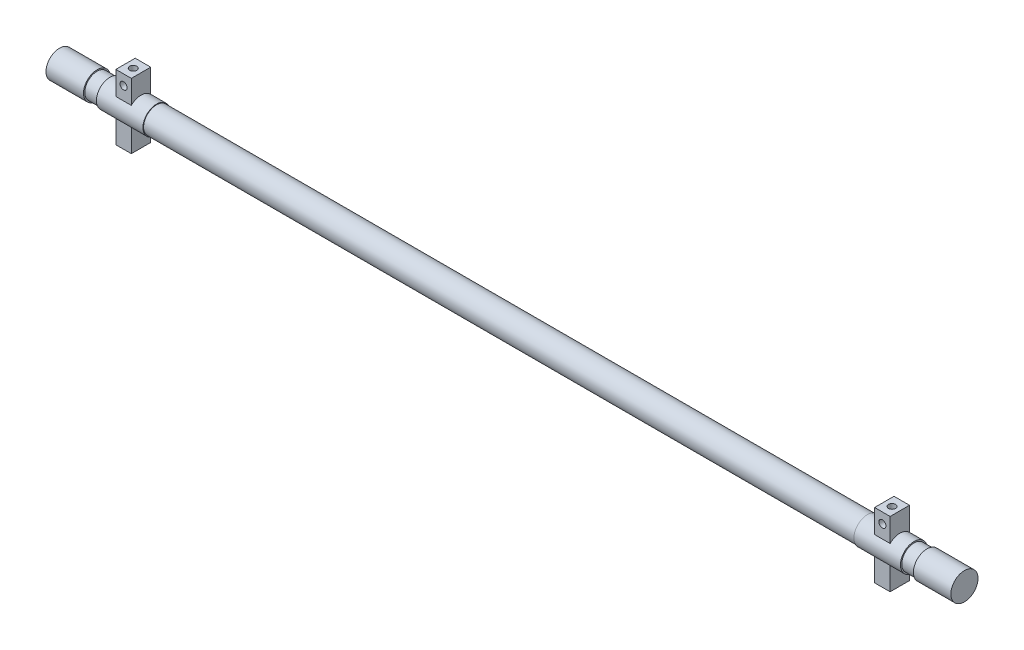
from build123d import *

# Parameters (mm, degrees)
SKETCH2_W            = 12
SKETCH2_H            = 35.5
BOSS_EXTRUDE1_DEPTH  = 7.5
LPATTERN1_COUNT      = 2
LPATTERN1_PITCH      = 587
BOSS_EXTRUDE2_DEPTH  = 15
M5_CLEARANCE_HOLE1_D = 5.5
M5_CLEARANCE_HOLE2_D = 5.5


with BuildPart() as part:
    # Sketch1 → Revolve1 (revolve)
    with BuildSketch(Plane.XY):
        Polygon((0, 0), (0, 10.5), (29, 10.5), (29, 9.5), (39, 9.5), (39, 10.5), (75, 10.5), (75, 10), (625, 10), (625, 10.5), (661, 10.5), (661, 9.5), (671, 9.5), (671, 10.5), (700, 10.5), (700, 0), align=None)
    revolve(axis=Axis((700, 0, 0), (-1, 0, 0)))

    # Sketch2 → Boss-Extrude1 (add, symmetric)
    with BuildSketch(Plane.XY):
        with Locations((57, -7.25)):
            Rectangle(SKETCH2_W, SKETCH2_H)
    boss_extrude1 = extrude(amount=BOSS_EXTRUDE1_DEPTH, both=True)

    # LPattern1: Boss-Extrude1 ×2
    with Locations(*[(i * LPATTERN1_PITCH, 0, 0) for i in range(1, LPATTERN1_COUNT)]):
        add(boss_extrude1)

    # Sketch3 → Boss-Extrude2 (add)
    with BuildSketch(Plane(origin=(0, 10.5, 0), x_dir=(1, 0, 0), z_dir=(0, 1, 0))):
        Polygon((63, -7.5), (63, 0), (63, 7.5), (51, 7.5), (51, 0), (51, -7.5), align=None)
        Polygon((650, -7.5), (650, 0), (650, 7.5), (638, 7.5), (638, 0), (638, -7.5), align=None)
    extrude(amount=BOSS_EXTRUDE2_DEPTH)

    # M5 Clearance Hole1 (through all)
    with Locations(Plane(origin=(0, 25.5, 0), x_dir=(1, 0, 0), z_dir=(0, 1, 0))):
        with Locations((57, 0), (644, 0)):
            Hole(M5_CLEARANCE_HOLE1_D / 2)

    # M5 Clearance Hole2 (through all)
    with Locations(Plane.XY.offset(7.5)):
        with Locations((57, 17.5), (644, 17.5)):
            Hole(M5_CLEARANCE_HOLE2_D / 2)


solid = part.part
